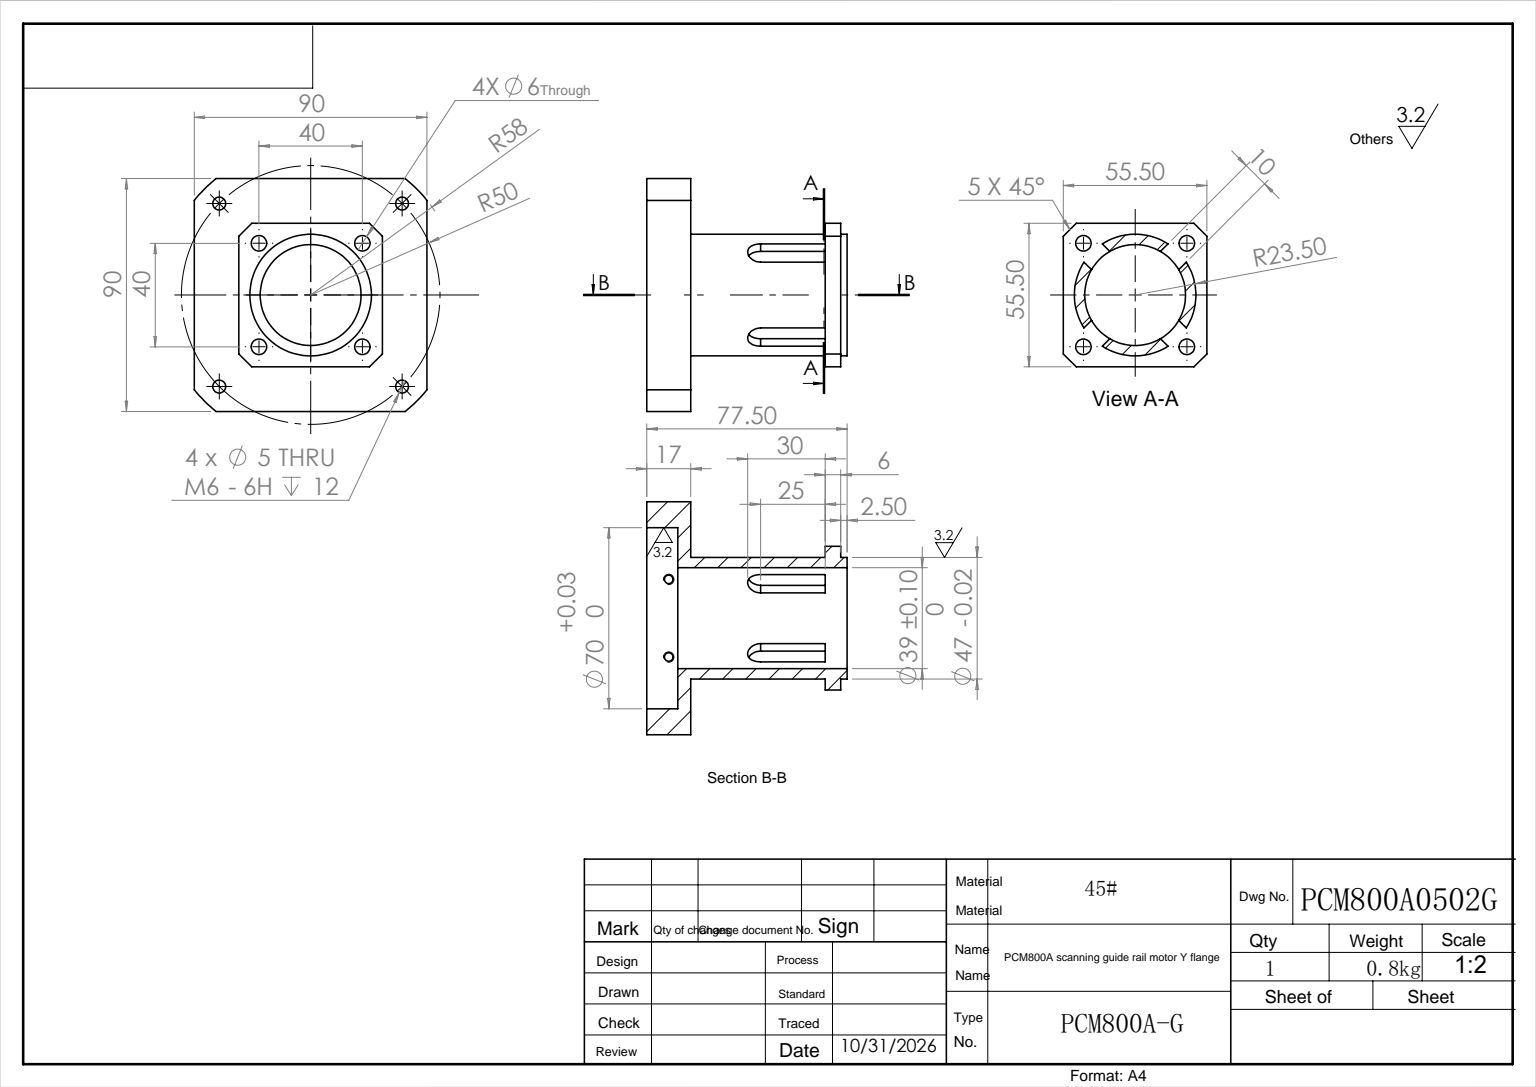
from build123d import *

# Parameters (mm, degrees)
SKETCH_1_W                   = 90
SKETCH_1_H                   = 90
EXTRUDE_1_DEPTH              = 17
SKETCH_2_R                   = 23.5
EXTRUDE_2_DEPTH              = 52
SKETCH_3_W                   = 55.5
SKETCH_3_H                   = 55.5
EXTRUDE_3_DEPTH              = 6
SKETCH_4_R                   = 23.5
EXTRUDE_4_DEPTH              = 2.5
SKETCH_5_R                   = 19.5
CUT_EXTRUDE_1_DEPTH          = 150.017616408
HOLE_WIZARD_M6_1_D           = 5
HOLE_WIZARD_M6_1_CBORE_D     = 6
HOLE_WIZARD_M6_1_CBORE_DEPTH = 12
SKETCH_8_R                   = 35
CUT_EXTRUDE_2_DEPTH          = 12
SKETCH_9_OUTSIDE_W           = 121.804
SKETCH_9_OUTSIDE_H           = 121.804
SKETCH_9_OUTSIDE_R           = 58
CUT_EXTRUDE_3_DEPTH          = 150.017616408
SKETCH_10_R                  = 3
CUT_EXTRUDE_4_DEPTH          = 12
CHAMFER_1_SIZE               = 5
CUT_EXTRUDE_5_DEPTH          = 146.62895586
CUT_EXTRUDE_6_DEPTH          = 118.175389983
HOLE_WIZARD_M4_1_REACH       = 142.926
HOLE_WIZARD_M4_1_BORE_R      = 1.65


with BuildPart() as part:
    # 草图1 → 拉伸1 (new body)
    with BuildSketch(Plane.XY):
        with Locations((45, 45)):
            Rectangle(SKETCH_1_W, SKETCH_1_H)
    extrude(amount=EXTRUDE_1_DEPTH)

    # 草图2 → 拉伸2 (add)
    with BuildSketch(Plane(origin=(0, 0, 0), x_dir=(-1, 0, 0), z_dir=(0, 0, -1))):
        with Locations(Location((-45, 45, 0), (0, 0, 180))):
            Circle(SKETCH_2_R)
    extrude(amount=EXTRUDE_2_DEPTH)

    # 草图3 → 拉伸3 (add)
    with BuildSketch(Plane(origin=(0, 0, -52), x_dir=(-1, 0, 0), z_dir=(0, 0, -1))):
        with Locations((-45, 45)):
            Rectangle(SKETCH_3_W, SKETCH_3_H)
    extrude(amount=EXTRUDE_3_DEPTH)

    # 草图4 → 拉伸4 (add)
    with BuildSketch(Plane(origin=(0, 0, -58), x_dir=(-1, 0, 0), z_dir=(0, 0, -1))):
        with Locations(Location((-45, 45, 0), (0, 0, 180))):
            Circle(SKETCH_4_R)
    extrude(amount=EXTRUDE_4_DEPTH)

    # 草图5 → 切除-拉伸1 (cut, through all)
    with BuildSketch(Plane(origin=(0, 0, -60.5), x_dir=(-1, 0, 0), z_dir=(0, 0, -1))):
        with Locations((-45, 45)):
            Circle(SKETCH_5_R)
    extrude(amount=-CUT_EXTRUDE_1_DEPTH, mode=Mode.SUBTRACT)

    # M6 螺纹孔1 (through all)
    with Locations(Plane(origin=(9.644660941, 80.355339059, 17), x_dir=(1, 0, 0), z_dir=(0, 0, 1))):
        with Locations((0, 0), (70.710678118, 0), (0, -70.710678118), (70.710678118, -70.710678118)):
            CounterBoreHole(HOLE_WIZARD_M6_1_D / 2, HOLE_WIZARD_M6_1_CBORE_D / 2, HOLE_WIZARD_M6_1_CBORE_DEPTH)

    # 草图8 → 切除-拉伸2 (cut)
    with BuildSketch(Plane.XY.offset(17)):
        with Locations((45, 45)):
            Circle(SKETCH_8_R)
    extrude(amount=-CUT_EXTRUDE_2_DEPTH, mode=Mode.SUBTRACT)

    # 草图9 outside → 切除-拉伸3 (cut, through all)
    with BuildSketch(Plane.XY.offset(17)):
        with Locations((45, 45)):
            Rectangle(SKETCH_9_OUTSIDE_W, SKETCH_9_OUTSIDE_H)
        with Locations((45, 45)):
            Circle(SKETCH_9_OUTSIDE_R, mode=Mode.SUBTRACT)
    extrude(amount=-CUT_EXTRUDE_3_DEPTH, mode=Mode.SUBTRACT)

    # 草图10 → 切除-拉伸4 (cut)
    with BuildSketch(Plane(origin=(0, 0, -58), x_dir=(-1, 0, 0), z_dir=(0, 0, -1))):
        with Locations((-65, 65)):
            Circle(SKETCH_10_R)
        with Locations((-25, 65)):
            Circle(SKETCH_10_R)
        with Locations((-25, 25)):
            Circle(SKETCH_10_R)
        with Locations((-65, 25)):
            Circle(SKETCH_10_R)
    extrude(amount=-CUT_EXTRUDE_4_DEPTH, mode=Mode.SUBTRACT)

    # 倒角1
    chamfer_1_edges = [part.edges().sort_by_distance(p)[0] for p in [
        (72.75, 72.75, -55),
        (72.75, 17.25, -55),
        (17.25, 17.25, -55),
        (17.25, 72.75, -55),
    ]]
    chamfer(chamfer_1_edges, length=CHAMFER_1_SIZE)

    # 草图11 → 切除-拉伸5 (cut, through all)
    with BuildSketch(Plane(origin=(-25.957106781, 25.957106781, 0), x_dir=(0, 0, 1), z_dir=(-0.7071067811865485, 0.7071067811865467, 0))):
        with BuildLine():
            Line((-52, 58.639610307), (-27, 58.639610307))
            ThreePointArc((-27, 58.639610307), (-22, 63.639610307), (-27, 68.639610307))
            Line((-27, 68.639610307), (-52, 68.639610307))
            Line((-52, 68.639610307), (-52, 58.639610307))
        make_face()
    extrude(amount=-CUT_EXTRUDE_5_DEPTH, mode=Mode.SUBTRACT)

    # 草图12 → 切除-拉伸6 (cut, through all)
    with BuildSketch(Plane(origin=(70.957106781, 70.957106781, 0), x_dir=(-0.7071067811865485, 0.7071067811865467, 0), z_dir=(0.7071067811865467, 0.7071067811865485, 0))):
        with BuildLine():
            Line((-5, -52), (5, -52))
            Line((5, -52), (5, -27))
            ThreePointArc((5, -27), (0, -22), (-5, -27))
            Line((-5, -27), (-5, -52))
        make_face()
    extrude(amount=-CUT_EXTRUDE_6_DEPTH, mode=Mode.SUBTRACT)

    # M4 螺纹孔1 bore → M4 螺纹孔1 (cut, up to next)
    with BuildSketch(Plane.XZ, mode=Mode.PRIVATE) as hole_wizard_m4_1_sk1:
        with Locations((60, 8.5)):
            Circle(HOLE_WIZARD_M4_1_BORE_R)
    hole_wizard_m4_1_tool1 = extrude(hole_wizard_m4_1_sk1.sketch, amount=-HOLE_WIZARD_M4_1_REACH, mode=Mode.PRIVATE) & part.part
    # M4 螺纹孔1 bore → M4 螺纹孔1 (cut, up to next)
    with BuildSketch(Plane.XZ, mode=Mode.PRIVATE) as hole_wizard_m4_1_sk2:
        with Locations((30, 8.5)):
            Circle(HOLE_WIZARD_M4_1_BORE_R)
    hole_wizard_m4_1_tool2 = extrude(hole_wizard_m4_1_sk2.sketch, amount=-HOLE_WIZARD_M4_1_REACH, mode=Mode.PRIVATE) & part.part
    add(hole_wizard_m4_1_tool1.solids().sort_by_distance((60, 0, 8.5))[0], mode=Mode.SUBTRACT)
    add(hole_wizard_m4_1_tool2.solids().sort_by_distance((30, 0, 8.5))[0], mode=Mode.SUBTRACT)


solid = part.part
